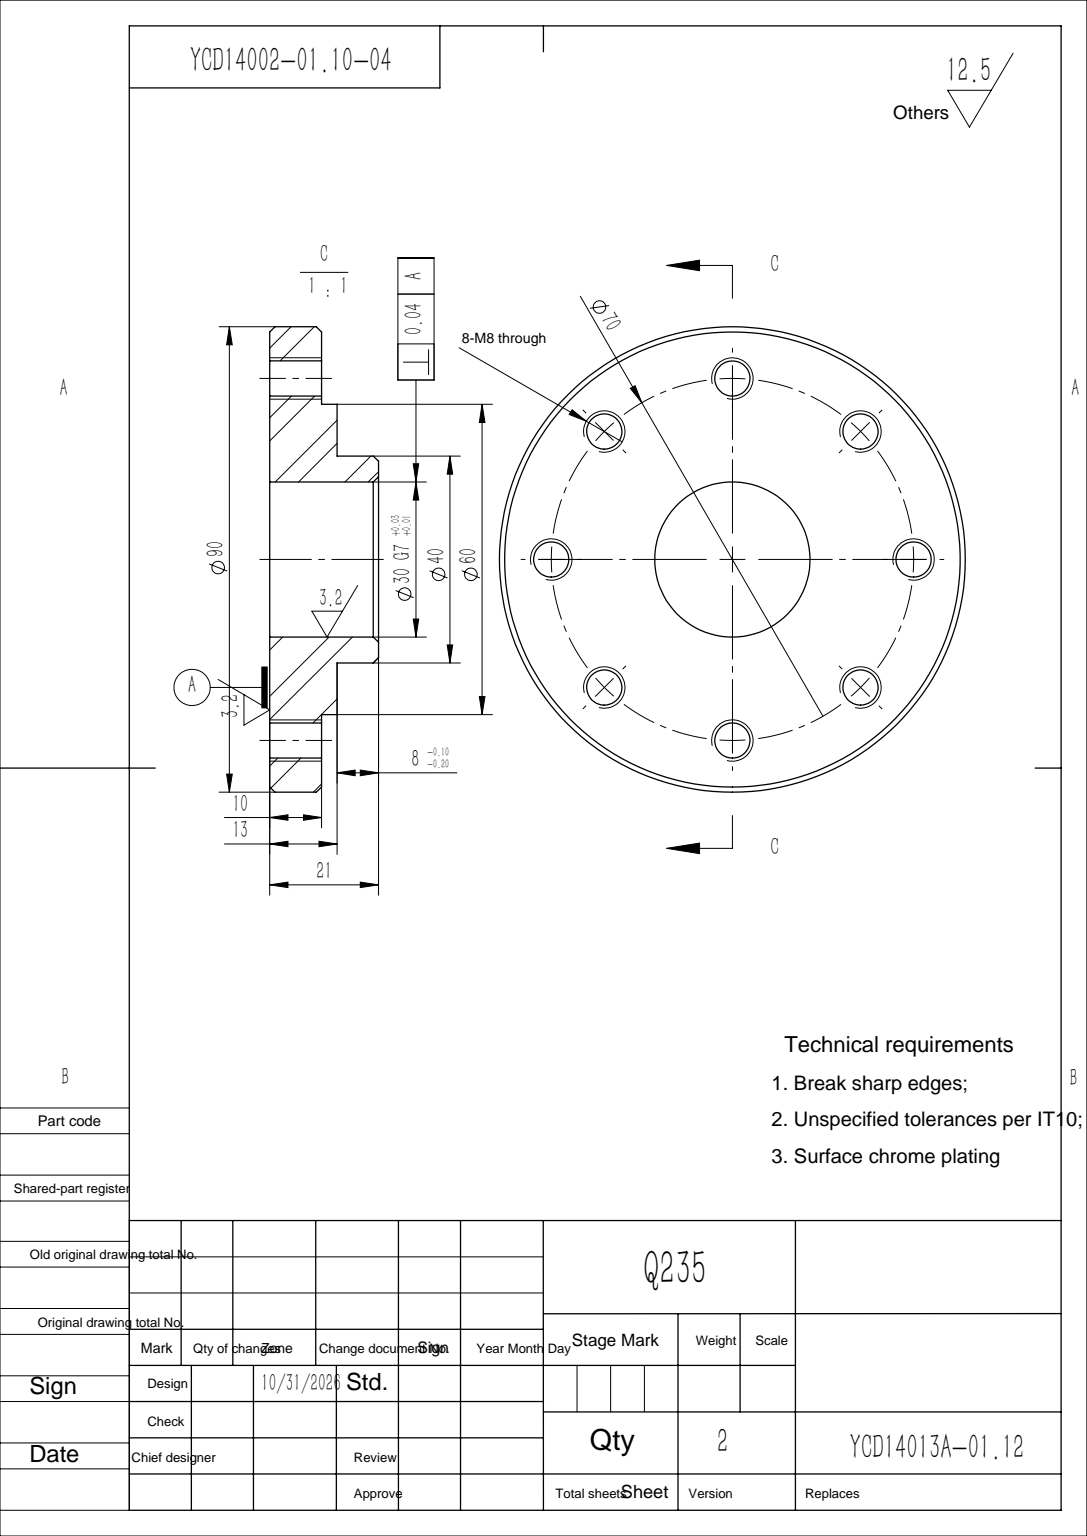
SolidWorks part; units mm, degrees
material "Q235"
ref_plane "Front Plane" through (0, 0, 0) normal (0, 0, 1) x (1, 0, 0)
ref_plane "Top Plane" through (0, 0, 0) normal (0, 1, 0) x (1, 0, 0)
ref_plane "Right Plane" through (0, 0, 0) normal (1, 0, 0) x (0, 0, -1)
sketch "Sketch1" plane through (0, 0, 0) normal (0, 1, 0) x (1, 0, 0)
  circle A0 centre (0, 0) radius 20
  dimension "D1" = 40
extrude "Boss-Extrude1" add sketch "Sketch1" along normal blind 8
sketch "Sketch3" plane through (0, 0, 0) normal (0, -1, 0) x (1, 0, 0)
  circle A0 centre (0, 0) radius 30
  dimension "D1" = 60
extrude "Boss-Extrude2" add sketch "Sketch3" along normal blind 3
sketch "Sketch4" plane through (0, -3, 0) normal (0, -1, 0) x (1, 0, 0)
  circle A0 centre (0, 0) radius 45
  dimension "D1" = 90
extrude "Boss-Extrude3" add sketch "Sketch4" along normal blind 10
sketch "Sketch5" plane through (0, 8, 0) normal (0, 1, 0) x (1, 0, 0)
  circle A0 centre (0, 0) radius 15
  dimension "D1" = 30
extrude "Cut-Extrude1" cut sketch "Sketch5" against normal blind 60
hole_wizard "Hole Size by Hex Socket Screw Type1" positions "Sketch8" profile "Sketch6" counterbore size "M8" standard "Gb"
sketch "Sketch8" plane through (0, -13, 0) normal (0, -1, 0) x (-1, 0, 0)
  point P0 (0, -9)
  dimension "D1" = 9
sketch "Sketch6" plane through (0, -13, 9) normal (1, 0, 0) x (0, 0, -1)
  line L0 (0, 0) -> (0, 21)
  line L1 (0, 21) -> (4.5, 21)
  line L3 (4.5, 21) -> (4.5, 9)
  line L4 (4.5, 9) -> (7.5, 9)
  line L5 (7.5, 9) -> (7.5, 0)
  line L7 (7.5, 0) -> (0, 0)
  line L11 (0, -6.35) -> (0, 107.95) construction
  dimension "通孔孔直径" = 9
  dimension "通孔孔深度" = 21
  dimension "柱形沉头孔直径" = 15
  dimension "柱形沉头孔深度" = 9
pattern_circular "CirPattern1" [suppressed] count 3 over 360
hole_wizard "M8 Tapped Hole1" positions "Sketch12" profile "Sketch13" tap size "M8" standard "Gb" end condition up to next
sketch "Sketch12" plane through (0, -13, 0) normal (0, -1, 0) x (-1, 0, 0)
  point P0 (0, -35)
  dimension "D1" = 35
sketch "Sketch13" plane through (0, -13, 35) normal (1, 0, 0) x (0, 0, -1)
  line L0 (0, 0) -> (0, 10.001)
  line L1 (0, 10.001) -> (3.4, 10.001)
  line L2 (3.4, 10.001) -> (3.4, 0)
  line L5 (3.4, 0) -> (0, 0)
  line L11 (0, -6.35) -> (0, 107.95) construction
  dimension "通孔螺纹孔钻头直径" = 6.8
  dimension "通孔螺纹孔钻头深度" = 10.001
cosmetic thread "Cosmetic Thread1" parameters "D2"=8
pattern_circular "CirPattern2" count 8 over 360 about axis through (0, 0, 0) along (0, 1, 0) of "M8 Tapped Hole1"
chamfer "Chamfer1" distance 1 angle 45 2 edges at (0, -3, -45) (0, -13, -45)
chamfer "Chamfer2" distance 1 angle 45 2 edges at (0, 8, 20) (0, 8, 15)
